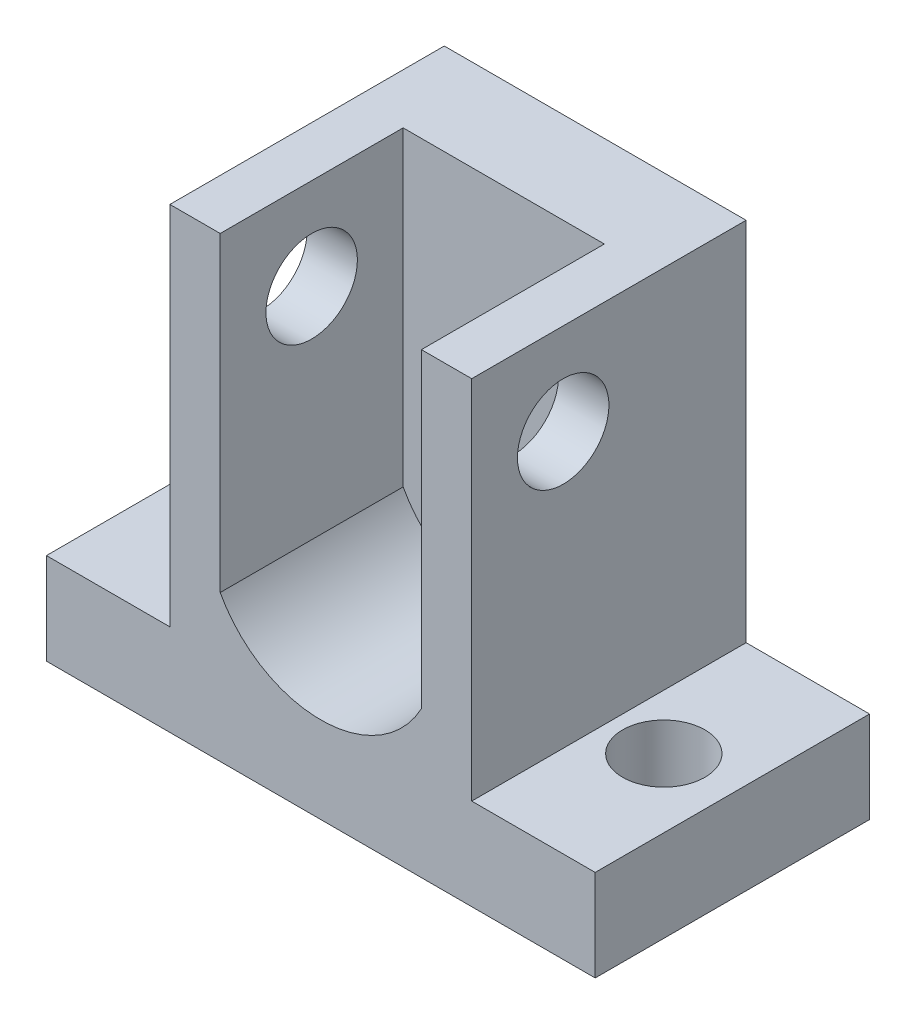
from build123d import *

# Parameters (mm, degrees)
SKETCH1_W                      = 60
SKETCH1_H                      = 50
BOSS_EXTRUDE1_DEPTH            = 30
SKETCH2_W                      = 13.5
SKETCH2_H                      = 40
CUT_EXTRUDE1_DEPTH             = 84.666002653
SKETCH3_W                      = 13.5
SKETCH3_H                      = 40
CUT_EXTRUDE2_DEPTH             = 84.666002653
CUT_EXTRUDE3_DEPTH             = 20
F_9_0_9_DIAMETER_HOLE1_D       = 9
F_10_0_10_DIAMETER_HOLE1_D     = 10
F_10_0_10_DIAMETER_HOLE1_DEPTH = 19
F_10_0_10_DIAMETER_HOLE2_D     = 10
F_10_0_10_DIAMETER_HOLE2_DEPTH = 19


with BuildPart() as part:
    # Sketch1 → Boss-Extrude1 (new body)
    with BuildSketch(Plane.XY.offset(30)):
        with Locations((30, 25)):
            Rectangle(SKETCH1_W, SKETCH1_H)
    extrude(amount=-BOSS_EXTRUDE1_DEPTH)

    # Sketch2 → Cut-Extrude1 (cut, through all)
    with BuildSketch(Plane(origin=(0, 0, 0), x_dir=(-1, 0, 0), z_dir=(0, 0, -1))):
        with Locations((-53.25, 30)):
            Rectangle(SKETCH2_W, SKETCH2_H)
    extrude(amount=-CUT_EXTRUDE1_DEPTH, mode=Mode.SUBTRACT)

    # Sketch3 → Cut-Extrude2 (cut, through all)
    with BuildSketch(Plane(origin=(0, 0, 0), x_dir=(-1, 0, 0), z_dir=(0, 0, -1))):
        with Locations((-6.75, 30)):
            Rectangle(SKETCH3_W, SKETCH3_H)
    extrude(amount=-CUT_EXTRUDE2_DEPTH, mode=Mode.SUBTRACT)

    # Sketch4 → Cut-Extrude3 (cut)
    with BuildSketch(Plane.XY.offset(30)):
        with BuildLine():
            Line((19, 50), (19, 16))
            ThreePointArc((19, 16), (30, 9.437171044), (41, 16))
            Line((41, 16), (41, 50))
            Line((41, 50), (19, 50))
        make_face()
    extrude(amount=-CUT_EXTRUDE3_DEPTH, mode=Mode.SUBTRACT)

    # Ø9.0 (9) Diameter Hole1 (through all)
    with Locations(Plane(origin=(0, 0, 0), x_dir=(-1, 0, 0), z_dir=(0, -1, 0))):
        with Locations((-7.5, -15), (-52.5, -15)):
            Hole(F_9_0_9_DIAMETER_HOLE1_D / 2)

    # Ø10.0 (10) Diameter Hole1
    with Locations(Plane.ZY.offset(-41)):
        with Locations((20, 40)):
            Hole(F_10_0_10_DIAMETER_HOLE1_D / 2, depth=F_10_0_10_DIAMETER_HOLE1_DEPTH)

    # Ø10.0 (10) Diameter Hole2
    with Locations(Plane(origin=(19, 0, 0), x_dir=(0, 0, -1), z_dir=(1, 0, 0))):
        with Locations((-20, 40)):
            Hole(F_10_0_10_DIAMETER_HOLE2_D / 2, depth=F_10_0_10_DIAMETER_HOLE2_DEPTH)


solid = part.part
